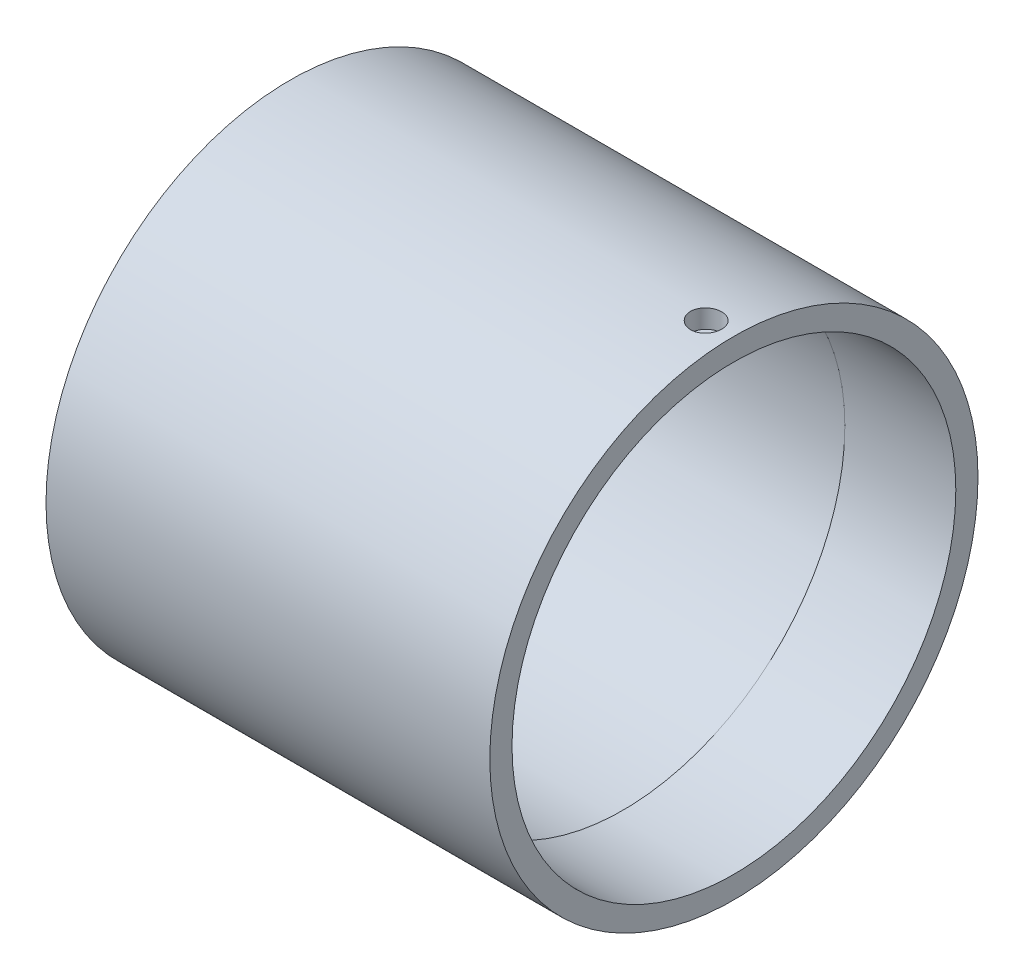
SolidWorks part; units mm, degrees
ref_plane "Front" through (0, 0, 0) normal (0, 0, 1) x (1, 0, 0)
ref_plane "Top" through (0, 0, 0) normal (0, 1, 0) x (1, 0, 0)
ref_plane "Right" through (0, 0, 0) normal (1, 0, 0) x (0, 0, -1)
sketch "Sketch2" plane through (0, 0, 0) normal (0, 0, 1) x (1, 0, 0)
  line L0 (-113.6297, 0) -> (137.4213, 0) construction
  line L1 (-80.9998, 110) -> (-80.9998, 100)
  line L2 (-80.9998, 110) -> (119.0002, 110)
  line L3 (119.0002, 110) -> (119.0002, 100)
  line L4 (119.0002, 100) -> (69.0002, 100)
  line L5 (69.0002, 100) -> (69.0002, 100.5)
  line L6 (69.0002, 100.5) -> (-53.9998, 100.5)
  line L7 (-53.9998, 100.5) -> (-53.9998, 100)
  line L8 (-53.9998, 100) -> (-63.4998, 100)
  line L9 (-63.4998, 100) -> (-63.4998, 105)
  line L10 (-63.4998, 105) -> (-70.9998, 105)
  line L11 (-70.9998, 105) -> (-70.9998, 100)
  line L12 (-80.9998, 100) -> (-70.9998, 100)
  dimension "D1" = 110
  dimension "D2" = 100
  dimension "D3" = 100.5
  dimension "D4" = 105
  dimension "D5" = 100
  dimension "D6" = 100
  dimension "D7" = 27
  dimension "D8" = 200
  dimension "D9" = 50
  dimension "D10" = 7.5
revolve "Revolve1" add sketch "Sketch2" angle 360 about L0
sketch "Sketch3" plane through (119.0002, 0, 0) normal (1, 0, 0) x (0, 0, -1)
  line L0 (0, 0) -> (0, 123.4228)
ref_plane "Plane1" through (0, 110, 0) normal (0, 1, 0) x (1, 0, 0)
sketch "Sketch4" plane through (0, 110, 0) normal (0, 1, 0) x (1, 0, 0)
  line L0 (119.0002, -110) -> (119.0002, 110) construction
  circle A0 centre (106.5002, 0) radius 7
  dimension "D1" = 12.5
  dimension "D2" = 14
extrude "Cut-Extrude1" cut sketch "Sketch4" against normal blind 8.5
sketch "Sketch5" plane through (0, 101.5, 0) normal (0, 1, 0) x (1, 0, 0)
  circle A0 centre (106.5002, 0) radius 4.25
  dimension "D1" = 8.5
extrude "Cut-Extrude2" cut sketch "Sketch5" against normal blind 8.5
equation "\"零件重量\"= IIF ( \"SW-质量\" > 100 , int ( \"SW-质量\" ) , \"SW-质量\" )"
